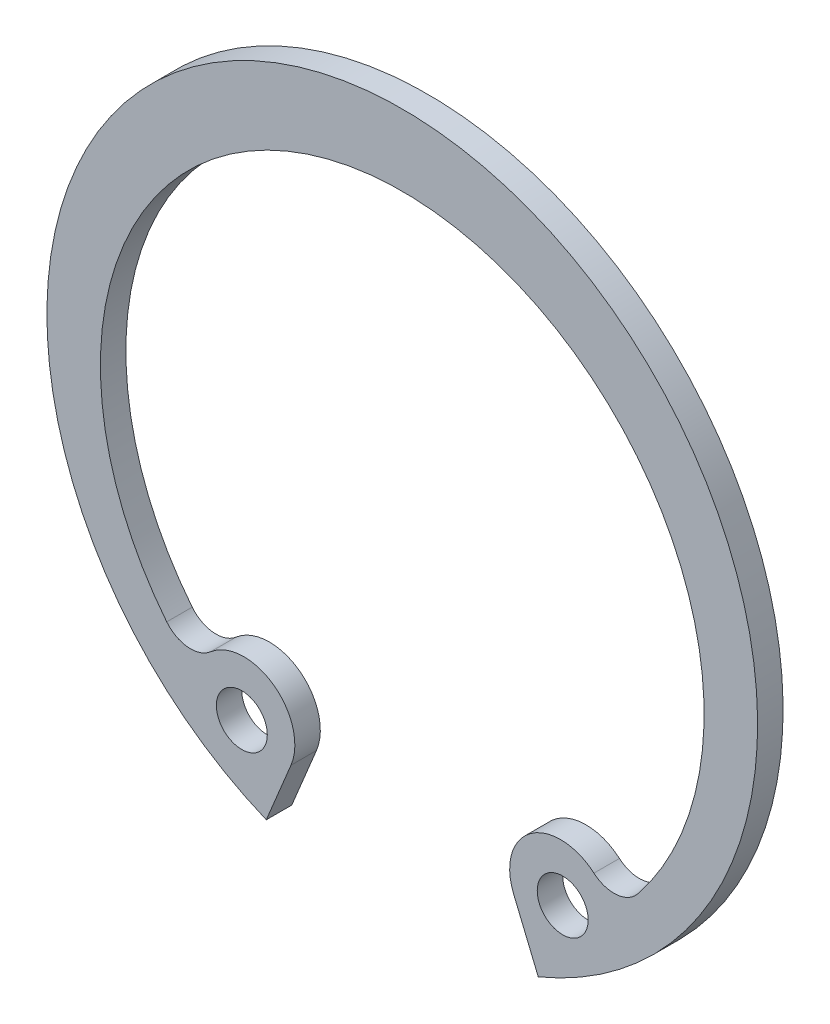
from build123d import *

# Parameters (mm, degrees)
SKETCH_1_R        = 1
EXTRUDE_967_DEPTH = 1


with BuildPart() as part:
    # 草图1 → Extrude 967 (new body)
    with BuildSketch(Plane.XY):
        with BuildLine():
            Line((-4.368765084, -10.547131916), (-5.338433881, -12.888119479))
            ThreePointArc((-5.338433881, -12.888119479), (0, 13.95), (5.338433881, -12.888119479))
            Line((5.338433881, -12.888119479), (4.368765084, -10.547131916))
            ThreePointArc((4.368765084, -10.547131916), (5.045920823, -8.160133818), (7.524722821, -8.268947735))
            ThreePointArc((7.524722821, -8.268947735), (8.418733826, -8.556288298), (9.245939718, -8.111821553))
            ThreePointArc((9.245939718, -8.111821553), (0, 11.15), (-9.245939718, -8.111821553))
            ThreePointArc((-9.245939718, -8.111821553), (-8.418733826, -8.556288298), (-7.524722821, -8.268947735))
            ThreePointArc((-7.524722821, -8.268947735), (-5.045920823, -8.160133818), (-4.368765084, -10.547131916))
        make_face()
        with Locations((-6.298089329, -9.978680815)):
            Circle(SKETCH_1_R, mode=Mode.SUBTRACT)
        with Locations(Location((6.298089329, -9.978680815, 0), (0, 0, 180))):
            Circle(SKETCH_1_R, mode=Mode.SUBTRACT)
    extrude(amount=EXTRUDE_967_DEPTH)


solid = part.part
